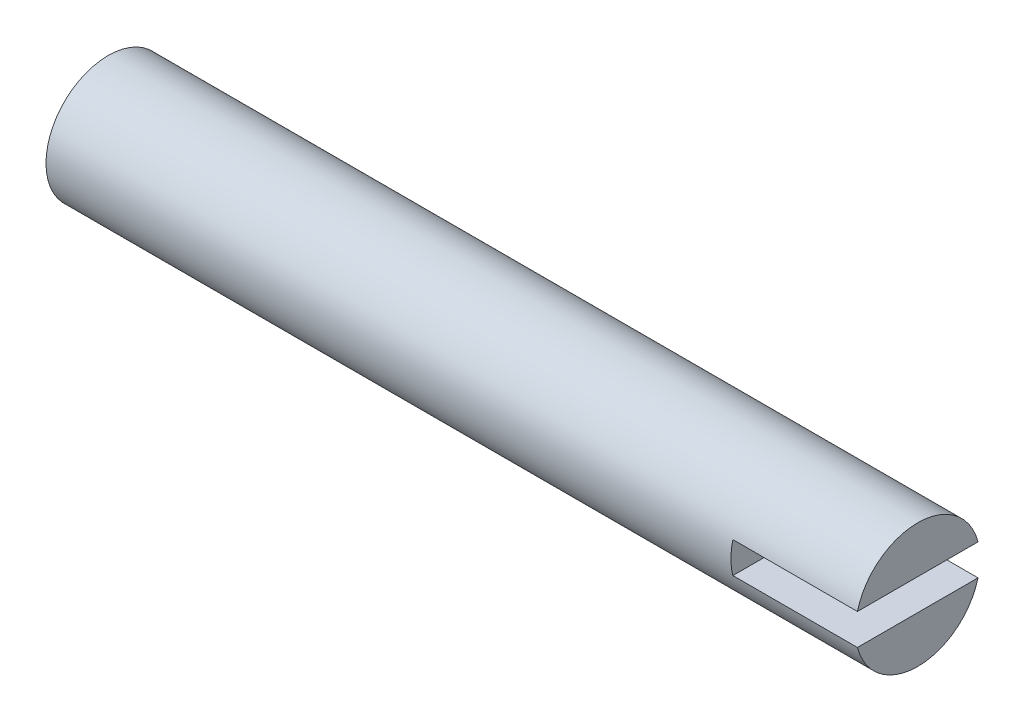
from build123d import *

# Parameters (mm, degrees)
SKETCH1_R           = 1
BOSS_EXTRUDE1_DEPTH = 13
SKETCH2_W           = 2.556803996
SKETCH2_H           = 0.5
CUT_EXTRUDE1_DEPTH  = 2


with BuildPart() as part:
    # Sketch1 → Boss-Extrude1 (new body)
    with BuildSketch(Plane(origin=(0, 0, 0), x_dir=(0, 0, -1), z_dir=(1, 0, 0))):
        with Locations(Location((0, 0, 0), (0, 0, 180))):
            Circle(SKETCH1_R)
    extrude(amount=BOSS_EXTRUDE1_DEPTH)

    # Sketch2 → Cut-Extrude1 (cut)
    with BuildSketch(Plane(origin=(13, 0, 0), x_dir=(0, 0, -1), z_dir=(1, 0, 0))):
        Rectangle(SKETCH2_W, SKETCH2_H)
    extrude(amount=-CUT_EXTRUDE1_DEPTH, mode=Mode.SUBTRACT)


solid = part.part
